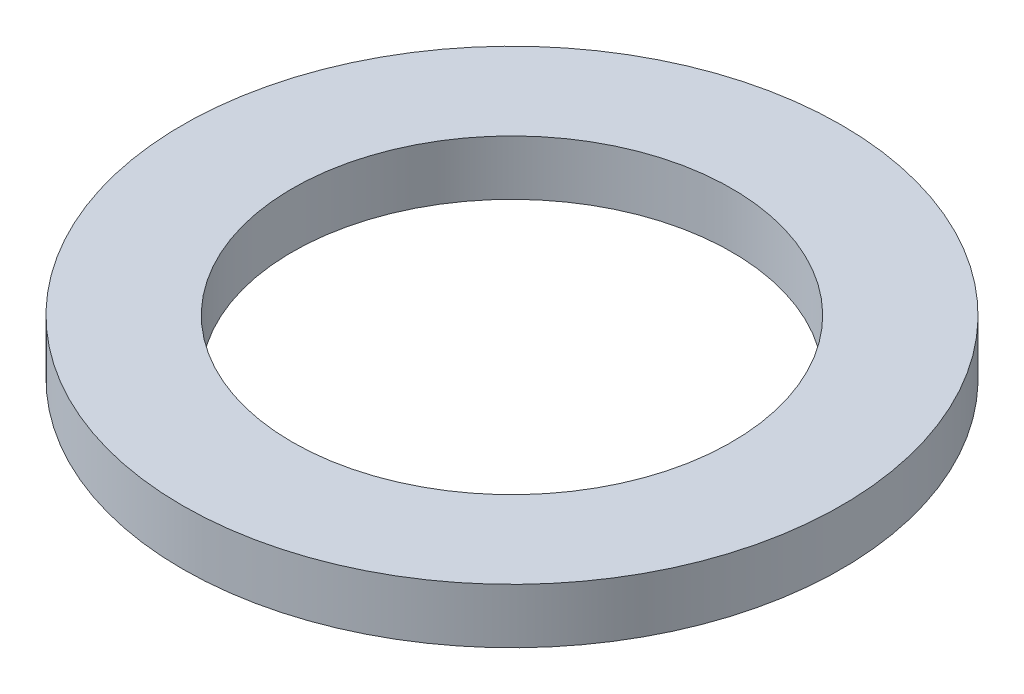
from build123d import *

# Parameters (mm, degrees)
SKETCH1_R           = 12
SKETCH1_R_2         = 8
BOSS_EXTRUDE3_DEPTH = 2


with BuildPart() as part:
    # Sketch1 → Boss-Extrude3 (new body)
    with BuildSketch(Plane(origin=(0, 0, 0), x_dir=(1, 0, 0), z_dir=(0, 1, 0))):
        with Locations(Location((0, 0, 0), (0, 0, 270))):
            Circle(SKETCH1_R)
        with Locations(Location((0, 0, 0), (0, 0, 270))):
            Circle(SKETCH1_R_2, mode=Mode.SUBTRACT)
    extrude(amount=BOSS_EXTRUDE3_DEPTH)


solid = part.part
